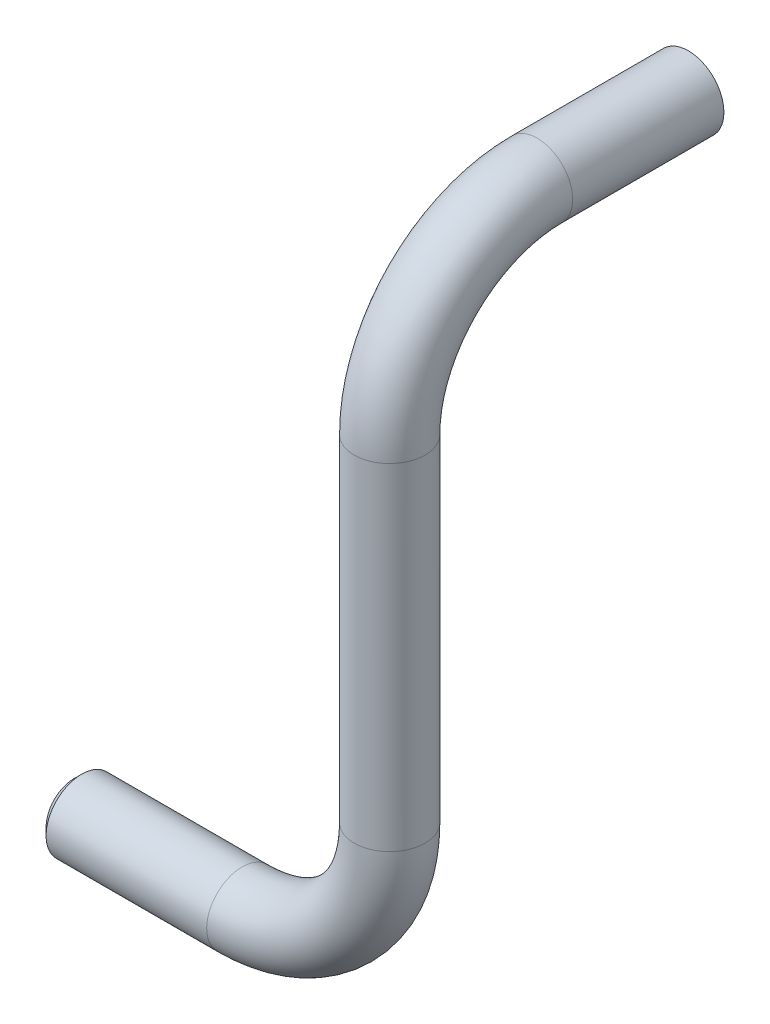
SolidWorks part; units mm, degrees
material "SS400B"
ref_plane "Front Plane" through (0, 0, 0) normal (0, 0, 1) x (1, 0, 0)
ref_plane "Top Plane" through (0, 0, 0) normal (0, 1, 0) x (1, 0, 0)
ref_plane "Right Plane" through (0, 0, 0) normal (1, 0, 0) x (0, 0, -1)
sketch3d "3DSketch1"
  line L0 (0, 0, 0) -> (0, 0, 40.5)
  line L1 (0, -39.5, 80) -> (0, -129.5, 80)
  line L2 (-39.5, -169, 80) -> (-84.5, -169, 80)
  arc A0 (0, -129.5, 80) -> (-39.5, -169, 80) centre (-39.5, -129.5, 80) ccw
  arc A1 (0, 0, 40.5) -> (0, -39.5, 80) centre (0, -39.5, 40.5) ccw
  point P7 (0, -169, 80)
  point P8 (-39.5, -129.5, 40.5)
  point P11 (0, 0, 80)
  point P12 (39.5, -39.5, 40.5)
  dimension "D4" = 39.5
  dimension "D1" = 80
  dimension "D2" = 169
  dimension "D3" = 84.5
sweep "Sweep1" add path "3DSketch1" circular profile diameter 19 parameters "D3"=19
chamfer "Chamfer1" distance 2 angle 45 1 edges at (-84.5, -169, 70.5)
